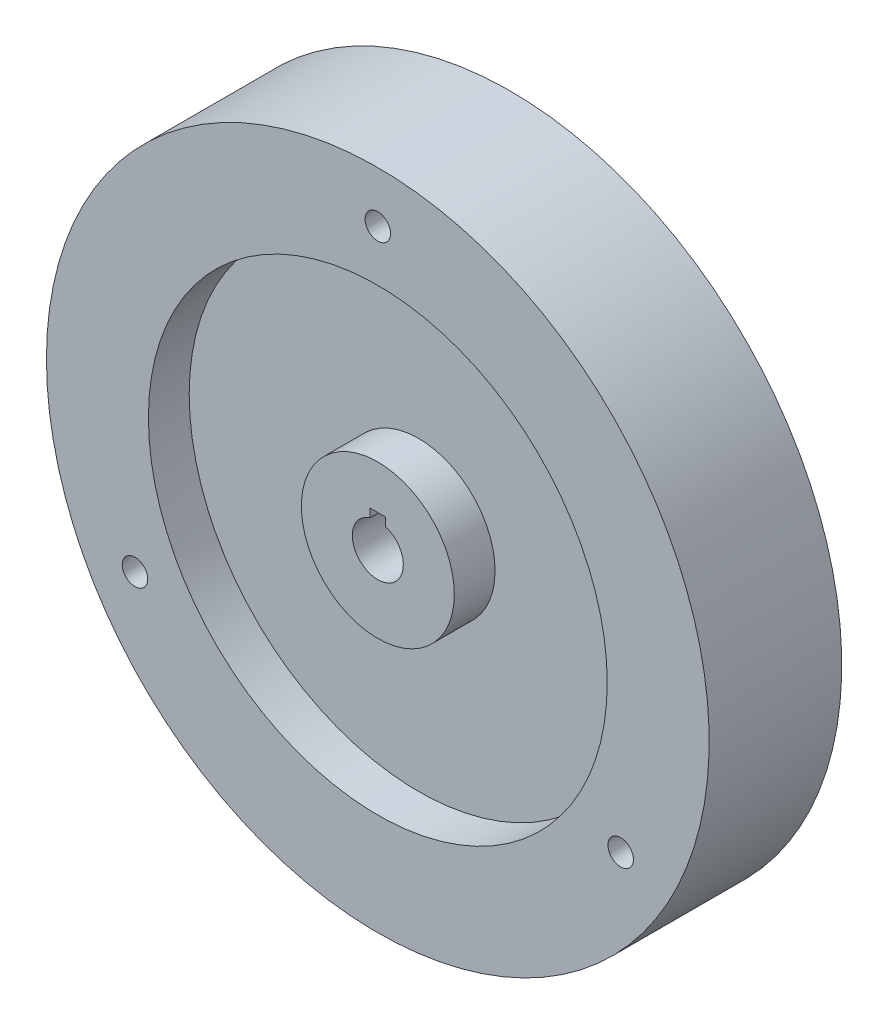
from build123d import *

# Parameters (mm, degrees)
SKETCH1_R           = 65
SKETCH1_R_2         = 2.5
BOSS_EXTRUDE1_DEPTH = 26
CUT_EXTRUDE1_DEPTH  = 96.530099969
SKETCH3_R           = 45
SKETCH3_R_2         = 15
CUT_EXTRUDE2_DEPTH  = 8
CUT_EXTRUDE3_START  = -8
SKETCH4_R           = 45
SKETCH4_R_2         = 15
CUT_EXTRUDE3_DEPTH  = 8


with BuildPart() as part:
    # Sketch1 → Boss-Extrude1 (new body)
    with BuildSketch(Plane.XY):
        with Locations(Location((0, 0, 0), (0, 0, 180))):
            Circle(SKETCH1_R)
        with Locations(Location((0, 55, 0), (0, 0, 180))):
            Circle(SKETCH1_R_2, mode=Mode.SUBTRACT)
        with Locations(Location((47.631397208, -27.5, 0), (0, 0, 180))):
            Circle(SKETCH1_R_2, mode=Mode.SUBTRACT)
        with Locations(Location((-47.631397208, -27.5, 0), (0, 0, 180))):
            Circle(SKETCH1_R_2, mode=Mode.SUBTRACT)
    extrude(amount=BOSS_EXTRUDE1_DEPTH)

    # Sketch2 → Cut-Extrude1 (cut, through all)
    with BuildSketch(Plane.XY.offset(26)):
        with BuildLine():
            Line((-1.5, 6.403418514), (1.5, 6.403418514))
            Line((1.5, 6.403418514), (1.5, 4.769696007))
            ThreePointArc((1.5, 4.769696007), (0, -5), (-1.5, 4.769696007))
            Line((-1.5, 4.769696007), (-1.5, 6.403418514))
        make_face()
    extrude(amount=-CUT_EXTRUDE1_DEPTH, mode=Mode.SUBTRACT)

    # Sketch3 → Cut-Extrude2 (cut)
    with BuildSketch(Plane.XY.offset(26)):
        Circle(SKETCH3_R)
        Circle(SKETCH3_R_2, mode=Mode.SUBTRACT)
    extrude(amount=-CUT_EXTRUDE2_DEPTH, mode=Mode.SUBTRACT)

    # Sketch4 → Cut-Extrude3 (cut)
    with BuildSketch(Plane(origin=(0, 0, 0), x_dir=(-1, 0, 0), z_dir=(0, 0, -1)).offset(CUT_EXTRUDE3_START)):
        with Locations(Location((0, 0, 0), (0, 0, 180))):
            Circle(SKETCH4_R)
        with Locations(Location((0, 0, 0), (0, 0, 180))):
            Circle(SKETCH4_R_2, mode=Mode.SUBTRACT)
    extrude(amount=CUT_EXTRUDE3_DEPTH, mode=Mode.SUBTRACT)


solid = part.part
